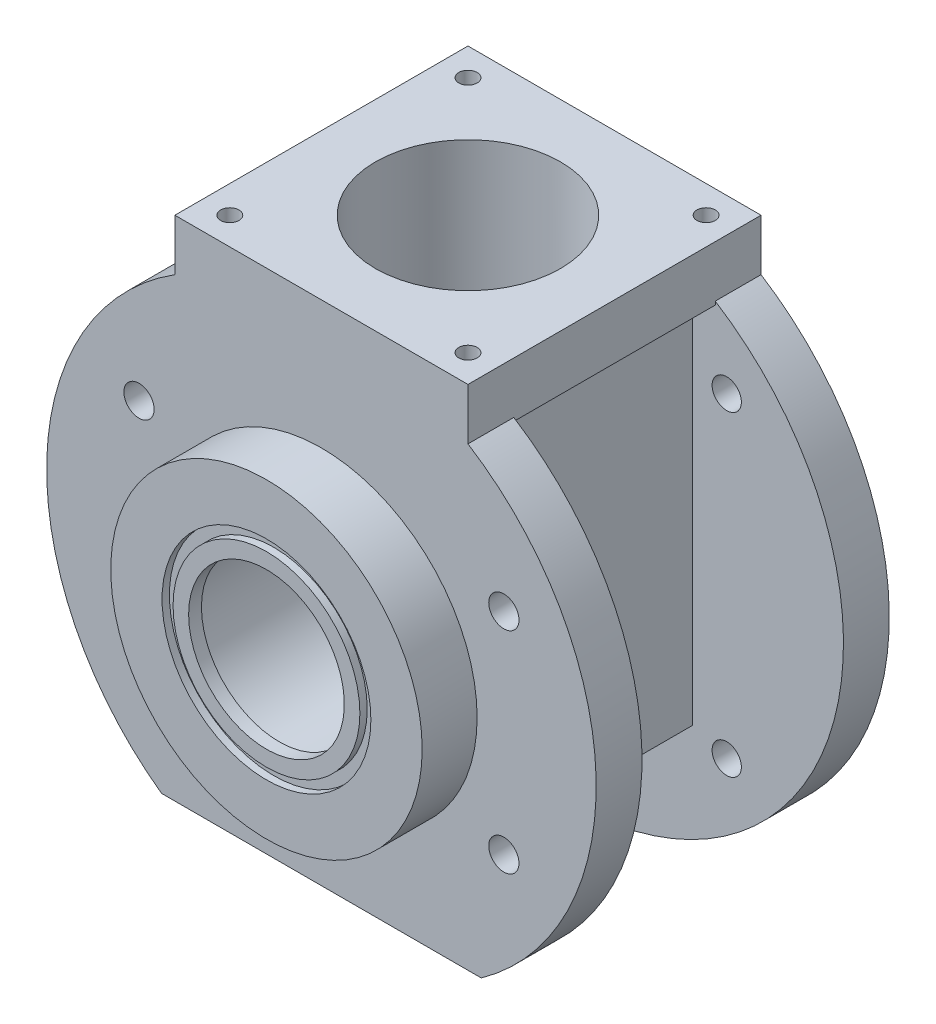
from build123d import *

# Parameters (mm, degrees)
BOSS_EXTRUDE1_DEPTH               = 25
SKETCH2_W                         = 160
SKETCH2_H                         = 206.885775404
BOSS_EXTRUDE2_DEPTH               = 110
BOSS_EXTRUDE3_DEPTH               = 25
SKETCH4_W                         = 160
SKETCH4_H                         = 160
BOSS_EXTRUDE4_DEPTH               = 28.114224596
CUT_EXTRUDE1_REACH                = 687.804
SKETCH6_W                         = 205
SKETCH6_H                         = 110
CUT_EXTRUDE2_REACH                = 894.915
SKETCH8_W                         = 12.5
SKETCH8_H                         = 110
SKETCH9_R                         = 85
BOSS_EXTRUDE5_DEPTH               = 30
HOLE1_D                           = 114
HOLE1_DEPTH                       = 4
SKETCH12_W                        = 110
SKETCH12_H                        = 8
SKETCH13_W                        = 51
SKETCH13_H                        = 4
F_16_0_16_DIAMETER_HOLE1_D        = 16
F_16_0_16_DIAMETER_HOLE1_DEPTH    = 25
F_16_5_16_5_DIAMETER_HOLE1_D      = 16.5
F_16_5_16_5_DIAMETER_HOLE1_DEPTH  = 55
F_10_0_10_DIAMETER_HOLE1_D        = 10
F_10_0_10_DIAMETER_HOLE1_DEPTH    = 30
F_8_0_8_DIAMETER_HOLE1_D          = 8
F_8_0_8_DIAMETER_HOLE1_DEPTH      = 18
M52_CLEARANCE_HOLE1_D             = 60
M52_CLEARANCE_HOLE1_DEPTH         = 40
M90_CLEARANCE_HOLE1_D             = 101
M90_CLEARANCE_HOLE1_DEPTH         = 155
M80_COUNTERBORE_HOLE1_D           = 85
M80_COUNTERBORE_HOLE1_CBORE_D     = 99
M80_COUNTERBORE_HOLE1_CBORE_DEPTH = 191


with BuildPart() as part:
    # Sketch1 → Boss-Extrude1 (new body)
    with BuildSketch(Plane(origin=(0, 0, -520.692981355), x_dir=(-1, 0, 0), z_dir=(0, 0, -1))):
        with BuildLine():
            Line((-441.230642584, 361.629739059), (-601.230642584, 361.629739059))
            ThreePointArc((-601.230642584, 361.629739059), (-521.230642584, 84.743963655), (-441.230642584, 361.629739059))
        make_face()
    extrude(amount=-BOSS_EXTRUDE1_DEPTH)

    # Sketch2 → Boss-Extrude2 (add)
    with BuildSketch(Plane.XY.offset(-495.692981355)):
        with Locations((521.230642584, 258.186851357)):
            Rectangle(SKETCH2_W, SKETCH2_H)
    extrude(amount=BOSS_EXTRUDE2_DEPTH)

    # Sketch3 → Boss-Extrude3 (add)
    with BuildSketch(Plane.XY.offset(-385.692981355)):
        with BuildLine():
            Line((608.500339501, 112.743963655), (433.960945667, 112.743963655))
            ThreePointArc((433.960945667, 112.743963655), (371.29458896, 239.123441208), (441.230642584, 361.629739059))
            Line((441.230642584, 361.629739059), (601.230642584, 361.629739059))
            ThreePointArc((601.230642584, 361.629739059), (671.166696208, 239.123441208), (608.500339501, 112.743963655))
        make_face()
    extrude(amount=BOSS_EXTRUDE3_DEPTH)

    # Sketch4 → Boss-Extrude4 (add)
    with BuildSketch(Plane(origin=(0, 361.629739059, 0), x_dir=(-1, 0, 0), z_dir=(0, 1, 0))):
        with Locations((-521.230642584, -440.692981355)):
            Rectangle(SKETCH4_W, SKETCH4_H)
    extrude(amount=BOSS_EXTRUDE4_DEPTH)

    # Sketch6 → Cut-Extrude1 (cut, up to next)
    with BuildSketch(Plane(origin=(588.730642584, 0, 0), x_dir=(0, -1, 0), z_dir=(-1, 0, 0)), mode=Mode.PRIVATE) as cut_extrude1_sk1:
        with Locations((-257.243963655, -440.692981355)):
            Rectangle(SKETCH6_W, SKETCH6_H)
    cut_extrude1_tool1 = extrude(cut_extrude1_sk1.sketch, amount=-CUT_EXTRUDE1_REACH, mode=Mode.PRIVATE) & part.part
    add(cut_extrude1_tool1.solids().sort_by_distance((588.730643, 257.243964, -440.692981))[0], mode=Mode.SUBTRACT)

    # Sketch8 → Cut-Extrude2 (cut, up to next)
    with BuildSketch(Plane(origin=(0, 359.743963655, 0), x_dir=(1, 0, 0), z_dir=(0, 1, 0)), mode=Mode.PRIVATE) as cut_extrude2_sk1:
        with Locations((447.480642584, 440.692981355)):
            Rectangle(SKETCH8_W, SKETCH8_H)
    cut_extrude2_tool1 = extrude(cut_extrude2_sk1.sketch, amount=-CUT_EXTRUDE2_REACH, mode=Mode.PRIVATE) & part.part
    add(cut_extrude2_tool1.solids().sort_by_distance((447.480643, 359.743964, -440.692981))[0], mode=Mode.SUBTRACT)

    # Sketch9 → Boss-Extrude5 (add)
    with BuildSketch(Plane.XY.offset(-360.692981355)):
        with Locations((521.230642584, 234.743963655)):
            Circle(SKETCH9_R)
    extrude(amount=BOSS_EXTRUDE5_DEPTH)

    # Hole1
    with Locations(Plane.XY.offset(-330.692981355)):
        with Locations((521.230642584, 234.743963655)):
            Hole(HOLE1_D / 2, depth=HOLE1_DEPTH)

    # Sketch12 → Revolve1 (revolve)
    with BuildSketch(Plane(origin=(0, 234.743963655, 0), x_dir=(1, 0, 0), z_dir=(0, 1, 0))):
        with Locations((576.230642584, 524.692981355)):
            Rectangle(SKETCH12_W, SKETCH12_H)
    revolve(axis=Axis((521.230642584, 234.743963655, -528.692981355), (0, 0, 1)))

    # Sketch13 → Revolve2 (revolve)
    with BuildSketch(Plane(origin=(0, 234.743963655, 0), x_dir=(1, 0, 0), z_dir=(0, 1, 0))):
        with Locations((546.730642584, 332.692981355)):
            Rectangle(SKETCH13_W, SKETCH13_H)
    revolve(axis=Axis((521.230642584, 234.743963655, -334.692981355), (0, 0, 1)))

    # Ø16.0 (16) diameter hole1
    with Locations(Plane(origin=(0, 0, -520.692981355), x_dir=(-1, 0, 0), z_dir=(0, 0, -1))):
        with Locations((-434.96361528, 321.010990959), (-607.497669889, 148.47693635), (-434.96361528, 148.47693635), (-607.497669889, 321.010990959)):
            Hole(F_16_0_16_DIAMETER_HOLE1_D / 2, depth=F_16_0_16_DIAMETER_HOLE1_DEPTH)

    # Ø16.5 (16.5) diameter hole1
    with Locations(Plane(origin=(0, 0, -385.692981355), x_dir=(-1, 0, 0), z_dir=(0, 0, -1))):
        with Locations((-620.82356402, 292.243963655), (-421.637721149, 177.243963655), (-421.637721149, 292.243963655), (-620.82356402, 177.243963655)):
            Hole(F_16_5_16_5_DIAMETER_HOLE1_D / 2, depth=F_16_5_16_5_DIAMETER_HOLE1_DEPTH)

    # Ø10.0 (10) diameter hole1
    with Locations(Plane(origin=(0, 389.743963655, 0), x_dir=(1, 0, 0), z_dir=(0, 1, 0))):
        with Locations((456.230642584, 505.692981355), (586.230642584, 505.692981355), (586.230642584, 375.692981355), (456.230642584, 375.692981355)):
            Hole(F_10_0_10_DIAMETER_HOLE1_D / 2, depth=F_10_0_10_DIAMETER_HOLE1_DEPTH)

    # Ø8.0 (8) diameter hole1
    with Locations(Plane(origin=(0, 154.743963655, 0), x_dir=(-1, 0, 0), z_dir=(0, -1, 0))):
        with Locations((-468.730642584, 480.692981355), (-573.730642584, 400.692981355), (-573.730642584, 480.692981355), (-468.730642584, 400.692981355)):
            Hole(F_8_0_8_DIAMETER_HOLE1_D / 2, depth=F_8_0_8_DIAMETER_HOLE1_DEPTH)

    # M52 clearance hole1
    with Locations(Plane(origin=(0, 154.743963655, 0), x_dir=(-1, 0, 0), z_dir=(0, -1, 0))):
        with Locations((-521.230642584, 440.692981355)):
            Hole(M52_CLEARANCE_HOLE1_D / 2, depth=M52_CLEARANCE_HOLE1_DEPTH)

    # M90 clearance hole1
    with Locations(Plane(origin=(0, 389.743963655, 0), x_dir=(1, 0, 0), z_dir=(0, 1, 0))):
        with Locations((521.230642584, 440.692981355)):
            Hole(M90_CLEARANCE_HOLE1_D / 2, depth=M90_CLEARANCE_HOLE1_DEPTH)

    # M80 counterbore hole1 (through all)
    with Locations(Plane(origin=(0, 0, -528.692981355), x_dir=(-1, 0, 0), z_dir=(0, 0, -1))):
        with Locations((-521.230642584, 234.743963655)):
            CounterBoreHole(M80_COUNTERBORE_HOLE1_D / 2, M80_COUNTERBORE_HOLE1_CBORE_D / 2, M80_COUNTERBORE_HOLE1_CBORE_DEPTH)


solid = part.part
